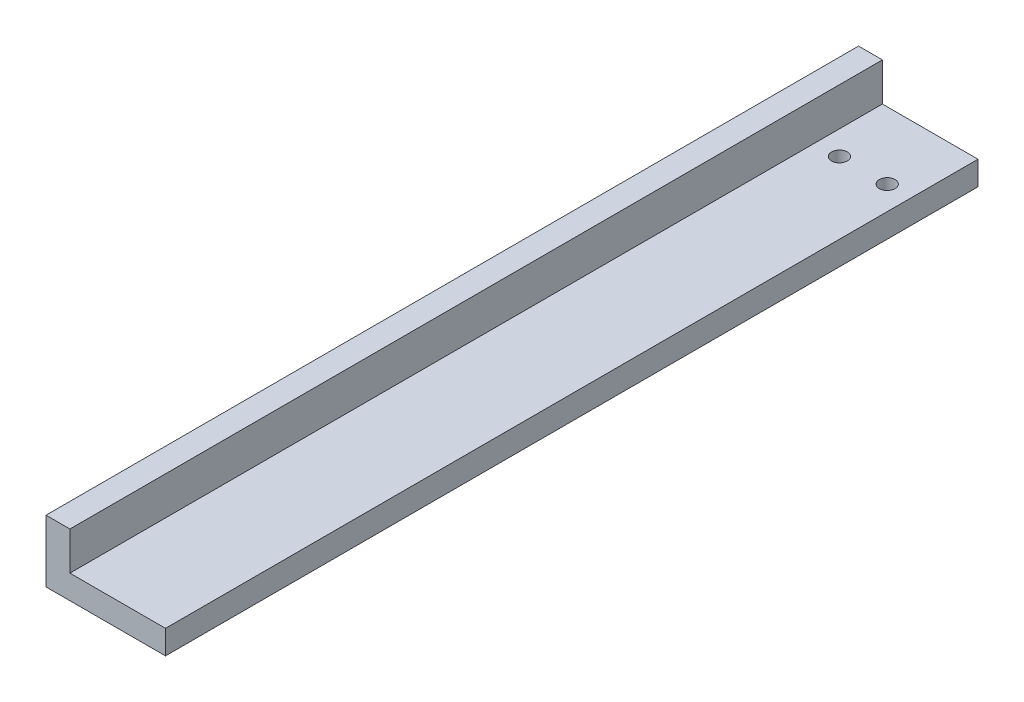
SolidWorks part; units mm, degrees
ref_plane "前视基准面" through (0, 0, 0) normal (0, 0, 1) x (1, 0, 0)
ref_plane "上视基准面" through (0, 0, 0) normal (0, 1, 0) x (1, 0, 0)
ref_plane "右视基准面" through (0, 0, 0) normal (1, 0, 0) x (0, 0, -1)
sketch "草图1" plane through (0, 0, 0) normal (0, 0, 1) x (1, 0, 0)
  line L0 (0, 0) -> (0, 13)
  line L1 (0, 13) -> (5, 13)
  line L2 (5, 13) -> (5, 5)
  line L3 (5, 5) -> (25, 5)
  line L4 (25, 5) -> (25, 0)
  line L5 (25, 0) -> (0, 0)
  dimension "D1" = 5
  dimension "D2" = 20
  dimension "D3" = 8
extrude "凸台-拉伸1" add sketch "草图1" along normal blind 170
hole_wizard "M4 螺纹孔1" positions "3D草图1" profile "草图2" tap size "M4" standard "GB" end condition up to next
sketch3d "3D草图1"
  line L0 (0, 0, 0) -> (25, 0, 0) construction
  line L1 (25, 0, 170) -> (25, 0, 0) construction
  point P0 (10, 0, 14)
  point P2 (20, 0, 14)
  dimension "D1" = 14
  dimension "D2" = 5
  dimension "D3" = 10
sketch "草图2" plane through (10, 0, 14) normal (1, 0, 0) x (0, 0, -1)
  line L0 (0, 0) -> (0, 5)
  line L1 (0, 5) -> (1.65, 5)
  line L2 (1.65, 5) -> (1.65, 0.375)
  line L3 (1.65, 0.375) -> (2.025, 0)
  line L5 (2.025, 0) -> (0, 0)
  line L6 (-1.65, 0.375) -> (-2.025, 0) construction
  line L11 (0, -6.35) -> (0, 107.95) construction
  dimension "通孔螺纹孔钻头直径" = 3.3
  dimension "通孔螺纹孔钻头深度" = 5
  dimension "近端锥形沉头孔直径" = 4.05
  dimension "近端锥形沉头孔角度" = 90
cosmetic thread "孔螺蚊线1"
cosmetic thread "孔螺蚊线2"
